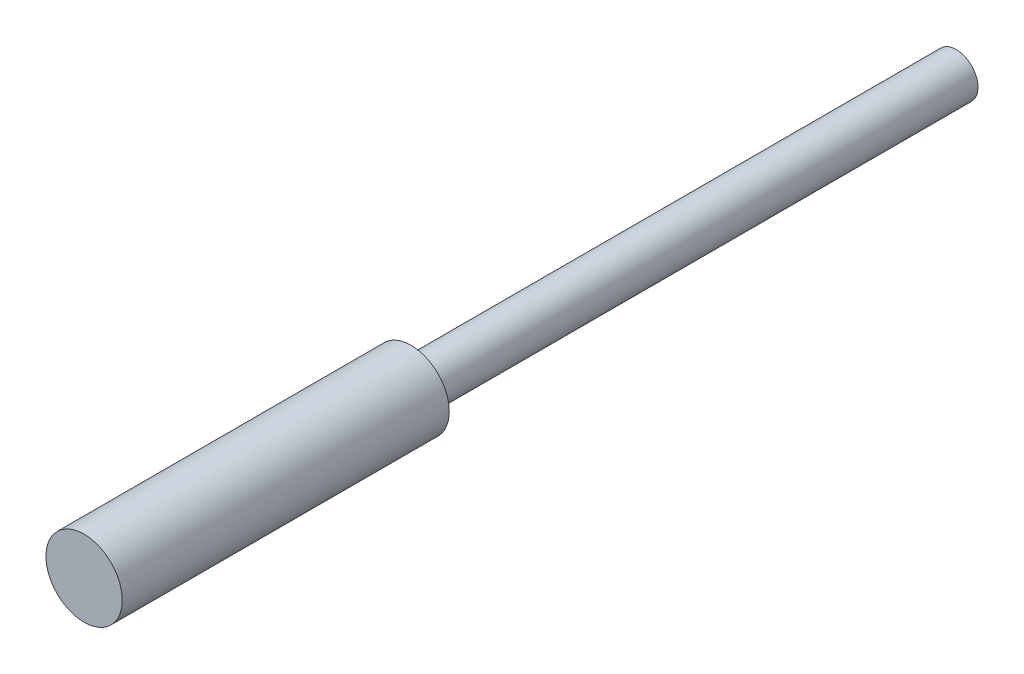
from build123d import *

# Parameters (mm, degrees)
SKETCH1_R           = 1.4
BOSS_EXTRUDE1_DEPTH = 12
SKETCH2_R           = 0.8
BOSS_EXTRUDE2_DEPTH = 20


with BuildPart() as part:
    # Sketch1 → Boss-Extrude1 (new body)
    with BuildSketch(Plane.XY):
        Circle(SKETCH1_R)
    extrude(amount=BOSS_EXTRUDE1_DEPTH)

    # Sketch2 → Boss-Extrude2 (add)
    with BuildSketch(Plane(origin=(0, 0, 0), x_dir=(-1, 0, 0), z_dir=(0, 0, -1))):
        with Locations(Location((0, 0, 0), (0, 0, 180))):
            Circle(SKETCH2_R)
    extrude(amount=BOSS_EXTRUDE2_DEPTH)


solid = part.part
